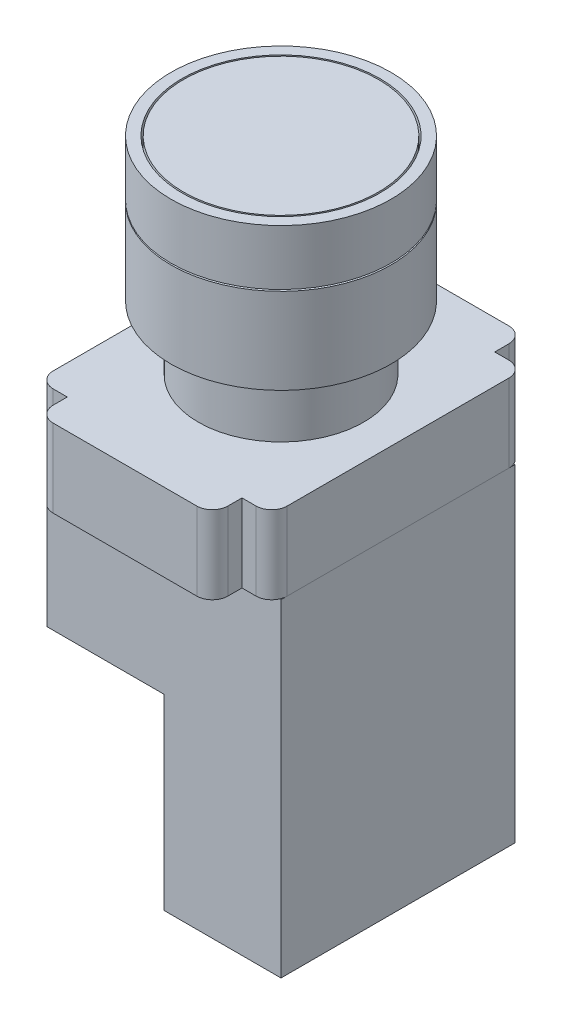
from build123d import *

# Parameters (mm, degrees)
SKETCH_2_W          = 30
SKETCH_2_H          = 40
EXTRUDE_1_DEPTH     = 10
SKETCH_3_W          = 15
SKETCH_3_H          = 30
EXTRUDE_2_DEPTH     = 42
SKETCH_7_W          = 3.8
SKETCH_7_H          = 3.8
CUT_EXTRUDE_2_DEPTH = 10
FILLET_1_R          = 2
SKETCH_8_W          = 15
SKETCH_8_H          = 30
EXTRUDE_3_DEPTH     = 18
SKETCH_11_W         = 1.4
SKETCH_11_H         = 7.1


with BuildPart() as part:
    # 草图1 → 旋转1 (revolve)
    with BuildSketch(Plane.XY, mode=Mode.PRIVATE) as revolve_1_sk:
        Polygon((12.5, 19.2), (14.1, 19.2), (14.1, 8.2), (10.6, 8.2), (10.6, 0), (0, 0), (0, 19.2), (0, 26.5), (12.5, 26.5), align=None)
    revolve(revolve_1_sk.sketch.rotate(Axis((0, 0, 0), (0, 1, 0)), 90), axis=Axis((0, 0, 0), (0, 1, 0)))


with BuildPart() as body_2:
    # 草图2 → 拉伸1 (new body)
    with BuildSketch(Plane.XZ):
        Rectangle(SKETCH_2_W, SKETCH_2_H)
    extrude(amount=EXTRUDE_1_DEPTH)

    # 草图7 → 切除-拉伸2 (cut)
    with BuildSketch(Plane(origin=(0, 0, 0), x_dir=(-1, 0, 0), z_dir=(0, 1, 0))):
        with Locations((-13.1, 18.1)):
            Rectangle(SKETCH_7_W, SKETCH_7_H)
        with Locations((13.1, 18.1)):
            Rectangle(SKETCH_7_W, SKETCH_7_H)
        with Locations((13.1, -18.1)):
            Rectangle(SKETCH_7_W, SKETCH_7_H)
        with Locations((-13.1, -18.1)):
            Rectangle(SKETCH_7_W, SKETCH_7_H)
    extrude(amount=-CUT_EXTRUDE_2_DEPTH, mode=Mode.SUBTRACT)

    # 圆角1
    fillet_1_edges = [body_2.edges().sort_by_distance(p)[0] for p in [
        (15, -5, 16.2),
        (11.2, -5, 20),
        (-11.2, -5, 20),
        (-15, -5, 16.2),
        (-15, -5, -16.2),
        (-11.2, -5, -20),
        (11.2, -5, -20),
        (15, -5, -16.2),
    ]]
    fillet(fillet_1_edges, radius=FILLET_1_R)


with BuildPart() as body_3:
    # 草图3 → 拉伸2 (new body)
    with BuildSketch(Plane.XZ.offset(10)):
        with Locations((7.5, 0)):
            Rectangle(SKETCH_3_W, SKETCH_3_H)
    extrude(amount=EXTRUDE_2_DEPTH)

    # 草图8 → 拉伸3 (add)
    with BuildSketch(Plane(origin=(0, -10, 0), x_dir=(-1, 0, 0), z_dir=(0, 1, 0))):
        with Locations((7.5, 0)):
            Rectangle(SKETCH_8_W, SKETCH_8_H)
    extrude(amount=-EXTRUDE_3_DEPTH)


with BuildPart() as body_4:
    # 草图11 → 旋转2 (revolve)
    with BuildSketch(Plane.XY, mode=Mode.PRIVATE) as revolve_2_sk:
        with Locations((13.4, 22.95)):
            Rectangle(SKETCH_11_W, SKETCH_11_H)
    revolve(revolve_2_sk.sketch.rotate(Axis((0, 0, 0), (0, 1, 0)), 90), axis=Axis((0, 0, 0), (0, 1, 0)))


solid = Compound([part.part, body_2.part, body_3.part, body_4.part])
